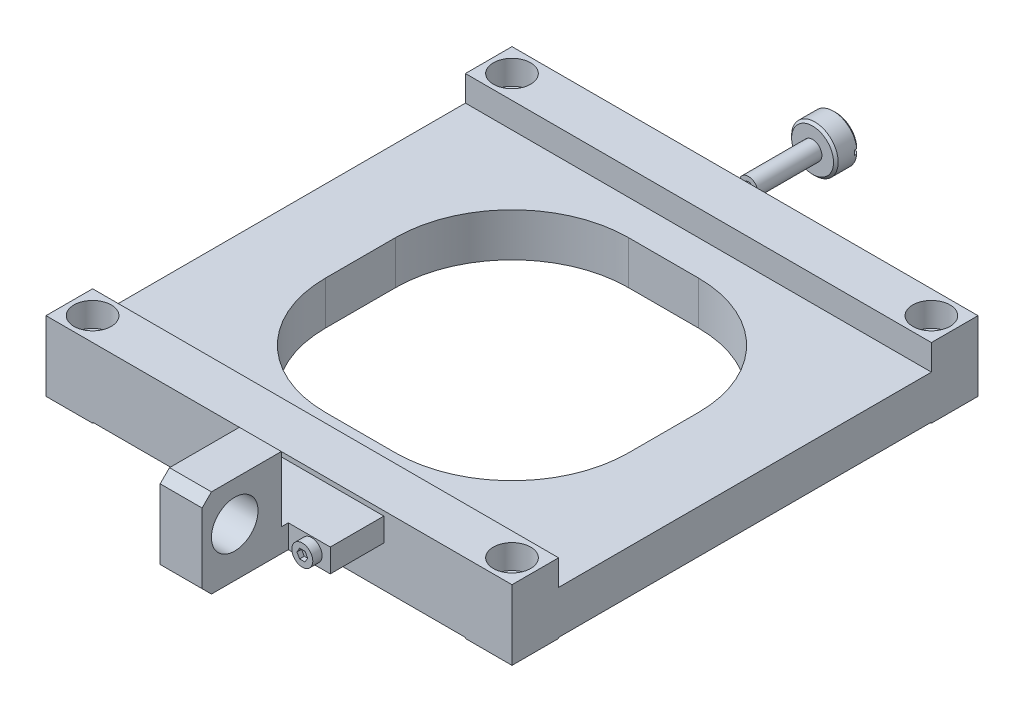
from build123d import *

# Parameters (mm, degrees)
EXTRUDE_1_DEPTH          = 50
EXTRUDE_1_DEPTH_BACK     = 50
CUT_EXTRUDE_1_DEPTH      = 50
CUT_EXTRUDE_1_DEPTH_BACK = 50
SKETCH_2_W               = 80
SKETCH_2_H               = 1
EXTRUDE_2_DEPTH          = 50
EXTRUDE_2_DEPTH_BACK     = 50
SKETCH_7_R               = 5
CUT_EXTRUDE_2_DEPTH      = 45
CUT_EXTRUDE_3_DEPTH      = 50
SKETCH_11_W              = 10
SKETCH_11_H              = 1
CUT_EXTRUDE_4_DEPTH      = 1
SKETCH_12_R              = 2.25
EXTRUDE_3_DEPTH          = 2
SKETCH_13_R              = 2.25
EXTRUDE_4_DEPTH          = 2
CUT_EXTRUDE_5_DEPTH      = 1
CUT_EXTRUDE_6_DEPTH      = 1


with BuildPart() as part:
    # 草图1 → 凸台-拉伸1 (new, two sides: drawn at the far end of the back side and taken through both)
    with BuildSketch(Plane(origin=(0, 0, 0), x_dir=(0, 0, -1), z_dir=(1, 0, 0)).offset(-EXTRUDE_1_DEPTH_BACK)):
        Polygon((-50, 15), (-50, 0), (-40, 0), (-40, 0.2), (40, 0.2), (40, 0), (50, 0), (50, 15), (40, 15), (40, 9.5), (-40, 9.5), (-40, 15), align=None)
    extrude(amount=EXTRUDE_1_DEPTH + EXTRUDE_1_DEPTH_BACK)

    # 草图2 → 切除-拉伸1 (cut, two sides: drawn at the far end of the back side and taken through both)
    with BuildSketch(Plane.XY.offset(-CUT_EXTRUDE_1_DEPTH_BACK)):
        with Locations((0, -0.3)):
            Rectangle(SKETCH_2_W, SKETCH_2_H)
    extrude(amount=CUT_EXTRUDE_1_DEPTH + CUT_EXTRUDE_1_DEPTH_BACK, mode=Mode.SUBTRACT)

    # 草图3 → 切除-旋转1 (revolve, cut)
    with BuildSketch(Plane(origin=(45, 0, 0), x_dir=(0, 0, -1), z_dir=(1, 0, 0)), mode=Mode.PRIVATE) as cut_revolve_1_sk:
        Polygon((-45, 15), (-41, 15), (-41, 9.8), (-42.75, 9.8), (-42.75, 0), (-45, 0), align=None)
    revolve(cut_revolve_1_sk.sketch.rotate(Axis((45, 0, 45), (0, 1, 0)), 180), axis=Axis((45, 0, 45), (0, 1, 0)), mode=Mode.SUBTRACT)

    # 草图4 → 切除-旋转2 (revolve, cut)
    with BuildSketch(Plane(origin=(-45, 0, 0), x_dir=(0, 0, -1), z_dir=(1, 0, 0)), mode=Mode.PRIVATE) as cut_revolve_2_sk:
        Polygon((-45, 15), (-41, 15), (-41, 9.8), (-42.75, 9.8), (-42.75, 0), (-45, 0), align=None)
    revolve(cut_revolve_2_sk.sketch.rotate(Axis((-45, 0, 45), (0, 1, 0)), 180), axis=Axis((-45, 0, 45), (0, 1, 0)), mode=Mode.SUBTRACT)

    # 草图5 → 切除-旋转3 (revolve, cut)
    with BuildSketch(Plane(origin=(-45, 0, 0), x_dir=(0, 0, -1), z_dir=(1, 0, 0)), mode=Mode.PRIVATE) as cut_revolve_3_sk:
        Polygon((45, 15), (49, 15), (49, 9.8), (47.25, 9.8), (47.25, 0), (45, 0), align=None)
    revolve(cut_revolve_3_sk.sketch.rotate(Axis((-45, 0, -45), (0, 1, 0)), 180), axis=Axis((-45, 0, -45), (0, 1, 0)), mode=Mode.SUBTRACT)

    # 草图6 → 切除-旋转4 (revolve, cut)
    with BuildSketch(Plane(origin=(45, 0, 0), x_dir=(0, 0, -1), z_dir=(1, 0, 0)), mode=Mode.PRIVATE) as cut_revolve_4_sk:
        Polygon((45, 15), (49, 15), (49, 9.8), (47.25, 9.8), (47.25, 0), (45, 0), align=None)
    revolve(cut_revolve_4_sk.sketch.rotate(Axis((45, 0, -45), (0, 1, 0)), 180), axis=Axis((45, 0, -45), (0, 1, 0)), mode=Mode.SUBTRACT)

    # 草图7 → 凸台-拉伸2 (add, two sides: drawn at the far end of the back side and taken through both)
    with BuildSketch(Plane(origin=(0, 0, 0), x_dir=(0, 0, -1), z_dir=(1, 0, 0)).offset(-EXTRUDE_2_DEPTH_BACK)):
        Polygon((-80, 26), (-80, 11), (-78, 9), (-50, 9), (-50, 14), (-63, 14), (-63, 28), (-78, 28), align=None)
        with Locations((-73, 19.5)):
            Circle(SKETCH_7_R, mode=Mode.SUBTRACT)
    extrude(amount=EXTRUDE_2_DEPTH + EXTRUDE_2_DEPTH_BACK)

    # 草图8 → 切除-拉伸2 (cut)
    with BuildSketch(Plane(origin=(0, 1, 0), x_dir=(-1, 0, 0), z_dir=(0, 1, 0))):
        Polygon((50, 84.5), (-50, 84.5), (-50, 50), (-22.5, 50), (-22.5, 61.5), (-13.5, 61.5), (-13.5, 81.8), (-4.5, 81.8), (-4.5, 61.5), (4.5, 61.5), (4.5, 50), (50, 50), align=None)
    extrude(amount=CUT_EXTRUDE_2_DEPTH, mode=Mode.SUBTRACT)

    # 草图9 → 旋转1 (revolve)
    with BuildSketch(Plane(origin=(0, 0, 0), x_dir=(0, 0, -1), z_dir=(1, 0, 0)), mode=Mode.PRIVATE) as revolve_1_sk:
        Polygon((50, 13.5), (50, 14.5), (50.75, 14.5), (50.75, 15.5), (64.5, 15.5), (64.5, 18), (65, 18.5), (69, 18.5), (69.5, 18), (69.5, 13.5), align=None)
    revolve(revolve_1_sk.sketch.rotate(Axis((0, 13.5, -69.5), (0, 0, 1)), 270), axis=Axis((0, 13.5, -69.5), (0, 0, 1)))

    # 草图10 → 切除-拉伸3 (cut)
    with BuildSketch(Plane(origin=(0, 0, 0), x_dir=(-1, 0, 0), z_dir=(0, 1, 0))):
        with BuildLine():
            Line((7.5, 32.5), (-7.5, 32.5))
            ThreePointArc((-7.5, 32.5), (-25.17766953, 25.17766953), (-32.5, 7.5))
            Line((-32.5, 7.5), (-32.5, -7.5))
            ThreePointArc((-32.5, -7.5), (-25.17766953, -25.17766953), (-7.5, -32.5))
            Line((-7.5, -32.5), (7.5, -32.5))
            ThreePointArc((7.5, -32.5), (25.17766953, -25.17766953), (32.5, -7.5))
            Line((32.5, -7.5), (32.5, 7.5))
            ThreePointArc((32.5, 7.5), (25.17766953, 25.17766953), (7.5, 32.5))
        make_face()
    extrude(amount=CUT_EXTRUDE_3_DEPTH, mode=Mode.SUBTRACT)

    # 草图11 → 切除-拉伸4 (cut)
    with BuildSketch(Plane(origin=(0, 0, -69.5), x_dir=(-1, 0, 0), z_dir=(0, 0, -1))):
        with Locations((0, 13.5)):
            Rectangle(SKETCH_11_W, SKETCH_11_H)
    extrude(amount=-CUT_EXTRUDE_4_DEPTH, mode=Mode.SUBTRACT)

    # 草图12 → 凸台-拉伸3 (add)
    with BuildSketch(Plane.XY.offset(61.5)):
        with Locations((-0.5, 11.5)):
            Circle(SKETCH_12_R)
    extrude(amount=EXTRUDE_3_DEPTH)

    # 草图13 → 凸台-拉伸4 (add)
    with BuildSketch(Plane.XY.offset(61.5)):
        with Locations((18.5, 11.5)):
            Circle(SKETCH_13_R)
    extrude(amount=EXTRUDE_4_DEPTH)

    # 草图14 → 切除-拉伸5 (cut)
    with BuildSketch(Plane.XY.offset(63.5)):
        Polygon((-1.077350269, 12.5), (-1.654700538, 11.5), (-1.077350269, 10.5), (0.077350269, 10.5), (0.654700538, 11.5), (0.077350269, 12.5), align=None)
    extrude(amount=-CUT_EXTRUDE_5_DEPTH, mode=Mode.SUBTRACT)

    # 草图15 → 切除-拉伸6 (cut)
    with BuildSketch(Plane.XY.offset(63.5)):
        Polygon((17.922649731, 12.5), (17.345299462, 11.5), (17.922649731, 10.5), (19.077350269, 10.5), (19.654700538, 11.5), (19.077350269, 12.5), align=None)
    extrude(amount=-CUT_EXTRUDE_6_DEPTH, mode=Mode.SUBTRACT)


solid = part.part
